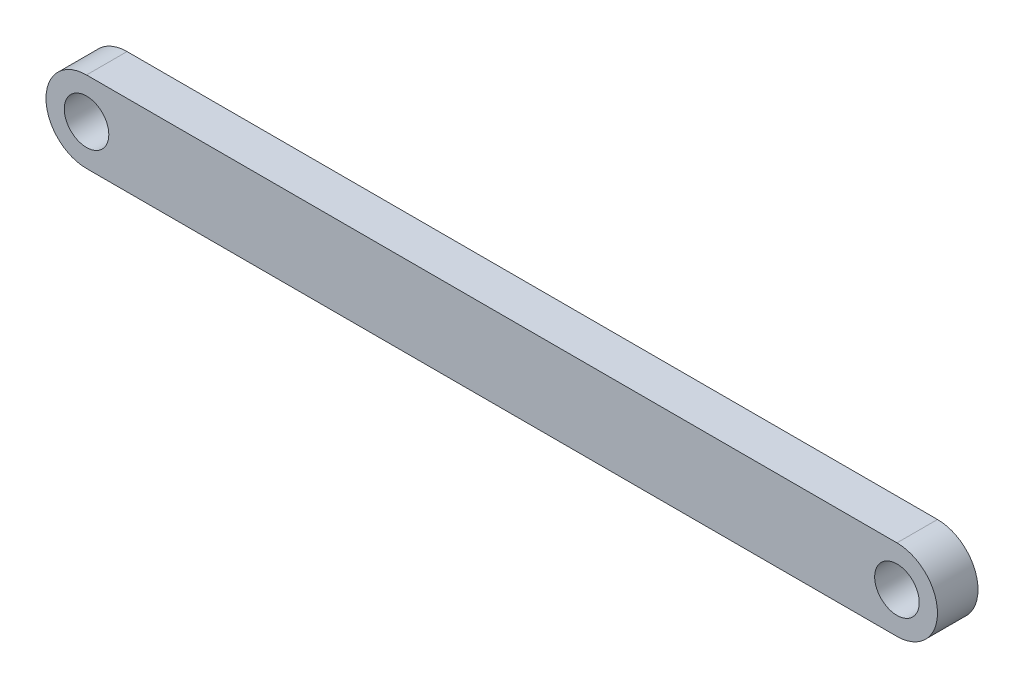
from build123d import *

# Parameters (mm, degrees)
SKETCH1_R           = 0.55
THIGH1_LENGTH_DEPTH = 0.5


with BuildPart() as part:
    # Sketch1 → Thigh1 length (new, symmetric)
    with BuildSketch(Plane.XY):
        with BuildLine():
            Line((-10, 1), (10, 1))
            ThreePointArc((10, 1), (11, 0), (10, -1))
            Line((10, -1), (-10, -1))
            ThreePointArc((-10, -1), (-11, 0), (-10, 1))
        make_face()
        with Locations((-10, 0)):
            Circle(SKETCH1_R, mode=Mode.SUBTRACT)
        with Locations((10, 0)):
            Circle(SKETCH1_R, mode=Mode.SUBTRACT)
    extrude(amount=THIGH1_LENGTH_DEPTH, both=True)


solid = part.part
